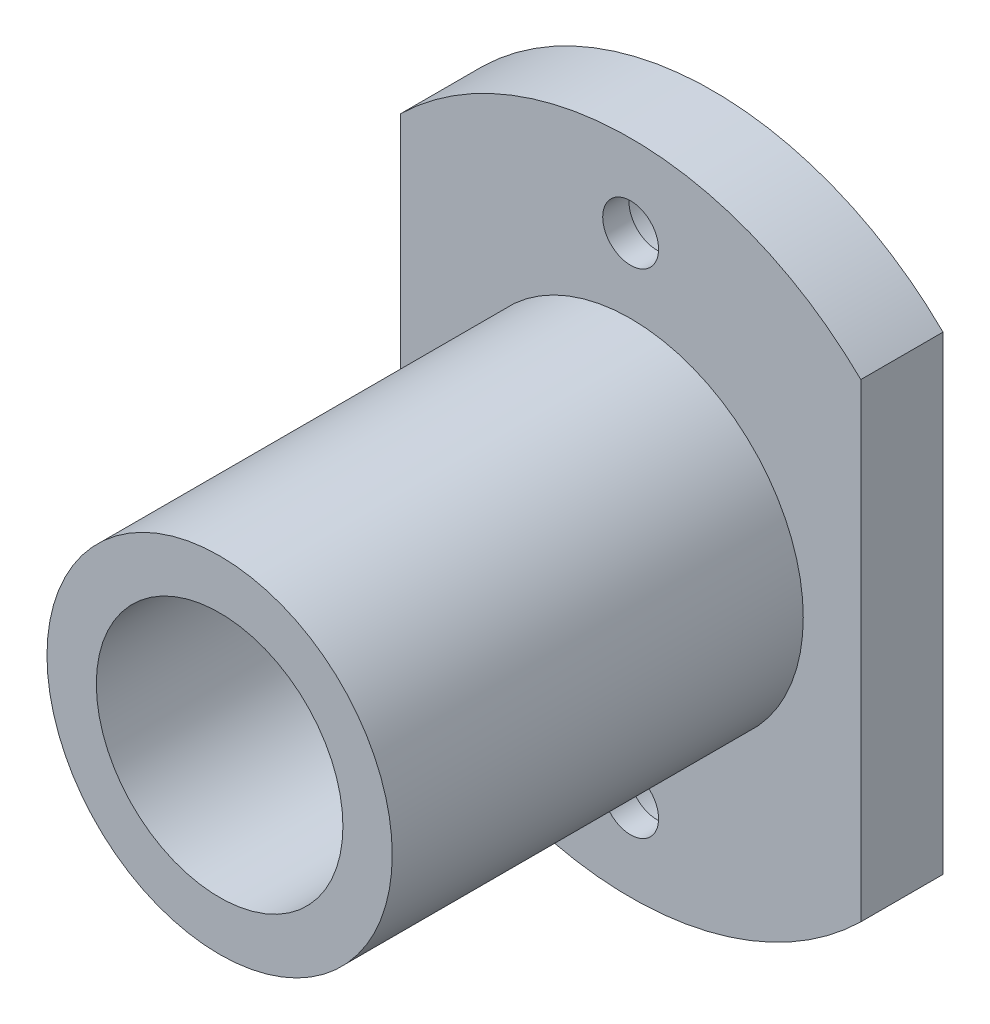
SolidWorks part; units mm, degrees
ref_plane "前视基准面" through (0, 0, 0) normal (0, 0, 1) x (1, 0, 0)
ref_plane "上视基准面" through (0, 0, 0) normal (0, 1, 0) x (1, 0, 0)
ref_plane "右视基准面" through (0, 0, 0) normal (1, 0, 0) x (0, 0, -1)
sketch "草图1" plane through (0, 0, 0) normal (0, 0, 1) x (1, 0, 0)
  circle A0 centre (0, 0) radius 7.5
  circle A1 centre (0, 0) radius 10.5
  dimension "D1" = 15
  dimension "D2" = 21
extrude "凸台-拉伸1" add sketch "草图1" along normal blind 25
sketch "草图3" plane through (0, 0, 0) normal (0, 0, -1) x (-1, 0, 0)
  circle A0 centre (0, 0) radius 7.5
  circle A1 centre (0, 0) radius 20
  dimension "D1" = 40
extrude "凸台-拉伸3" add sketch "草图3" along normal blind 5
hole_wizard "打孔尺寸根据内六角圆柱头螺钉的类型1" positions "草图5" profile "草图4" counterbore size "M3" standard "Gb" end condition through all
sketch "草图5" plane through (0, 0, -5) normal (0, 0, -1) x (-1, 0, 0)
  line L0 (0, 15) -> (0, -15) construction
  point P0 (0, 15)
  point P2 (0, -15)
  point P9 (0, 0)
  dimension "D1" = 30
sketch "草图4" plane through (0, 15, -5) normal (1, 0, 0) x (0, 1, 0)
  line L0 (0, 0) -> (0, 30)
  line L1 (0, 30) -> (1.7, 30)
  line L3 (1.7, 30) -> (1.7, 3.4)
  line L4 (1.7, 3.4) -> (3, 3.4)
  line L5 (3, 3.4) -> (3, 0)
  line L7 (3, 0) -> (0, 0)
  line L11 (0, -6.35) -> (0, 107.95) construction
  dimension "通孔孔直径" = 3.4
  dimension "通孔孔深度" = 30
  dimension "柱形沉头孔直径" = 6
  dimension "柱形沉头孔深度" = 3.4
sketch "草图6" plane through (0, 0, -5) normal (0, 0, -1) x (-1, 0, 0)
  line L1 (-24.7264, 22.5933) -> (-14, 22.5933)
  line L2 (-24.7264, 22.5933) -> (-24.7264, -17.9182)
  line L3 (-24.7264, -17.9182) -> (-14, -17.9182)
  line L4 (-14, 22.5933) -> (-14, -17.9182)
  line L5 (21.8533, 20.4863) -> (14, 20.4863)
  line L6 (21.8533, 20.4863) -> (21.8533, -22.2279)
  line L7 (21.8533, -22.2279) -> (14, -22.2279)
  line L8 (14, 20.4863) -> (14, -22.2279)
  dimension "D1" = 14
  dimension "D2" = 14
extrude "切除-拉伸1" cut sketch "草图6" against normal blind 10
